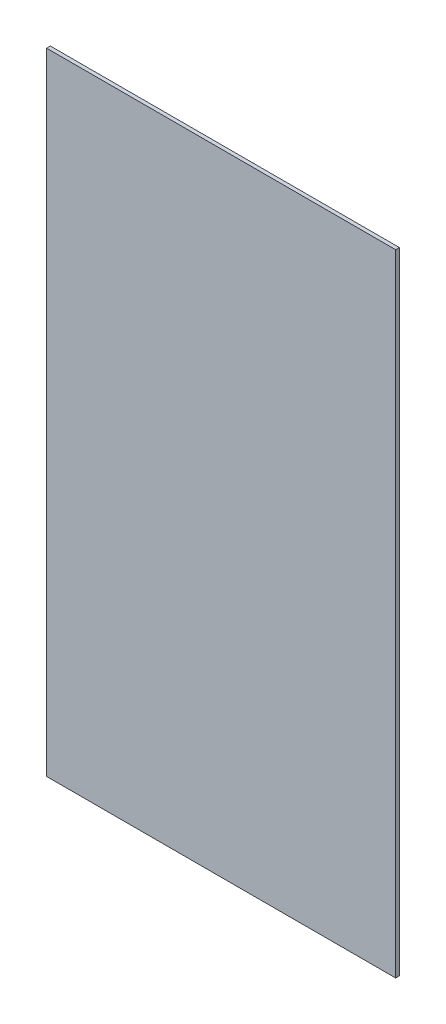
SolidWorks part; units mm, degrees
material "PMMA(有机玻璃)"
ref_plane "前视" through (0, 0, 0) normal (0, 0, 1) x (1, 0, 0)
ref_plane "上视" through (0, 0, 0) normal (0, 1, 0) x (1, 0, 0)
ref_plane "右视" through (0, 0, 0) normal (1, 0, 0) x (0, 0, -1)
sketch "草图1" plane through (0, 0, 0) normal (0, 0, 1) x (1, 0, 0)
  line L1 (-233, 421) -> (233, 421)
  line L2 (-233, 421) -> (-233, -421)
  line L3 (-233, -421) -> (233, -421)
  line L4 (233, 421) -> (233, -421)
  line L5 (-233, 421) -> (233, -421) construction
  line L6 (-233, -421) -> (233, 421) construction
  point P0 (0, 0)
  dimension "D1" = 842
  dimension "D2" = 466
extrude "凸台-拉伸1" add sketch "草图1" along normal blind 5
hole_wizard "M5 间隙孔1" positions "草图3" profile "草图2" hole size "M5" standard "GB"
sketch "草图3" plane through (0, 0, 5) normal (0, 0, 1) x (1, 0, 0)
  line L0 (-427.5, 273) -> (-427.5, -273) construction
  line L1 (-427.5, -273) -> (427.5, -273) construction
  line L2 (0, 273) -> (0, -273) construction
  line L3 (427.5, 273) -> (-427.5, 273) construction
  line L5 (-427.5, 0) -> (427.5, 0) construction
  line L6 (427.5, -273) -> (427.5, 273) construction
  point P0 (-375, -261)
  point P46 (415.5, 250)
  point P48 (-415.5, 250)
  point P58 (-125, -261)
  point P59 (125, -261)
  point P61 (-125, 261)
  point P62 (125, 261)
  point P64 (-375, 261)
  point P88 (375, -261)
  point P89 (375, 261)
  point P108 (415.5, 0)
  point P109 (-415.5, 0)
  point P110 (415.5, -250)
  point P111 (-415.5, -250)
  dimension "D1" = 12
  dimension "D2" = 12
  dimension "D5" = 3
  dimension "D3" = 12
  dimension "D6" = 4
  dimension "D4" = 2
sketch "草图2" plane through (-375, -261, 5) normal (1, 0, 0) x (0, -1, 0)
  line L0 (0, 0) -> (0, 5)
  line L1 (0, 5) -> (2.75, 5)
  line L2 (2.75, 5) -> (2.75, 0)
  line L5 (2.75, 0) -> (0, 0)
  line L11 (0, -6.35) -> (0, 107.95) construction
  dimension "通孔孔直径" = 5.5
  dimension "通孔孔深度" = 5
